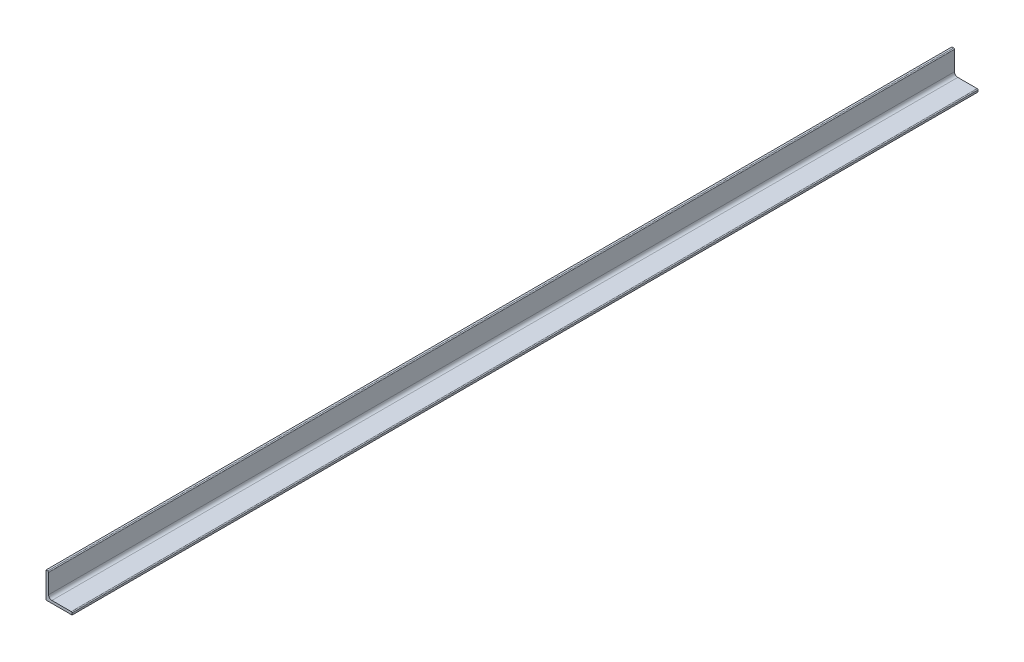
from build123d import *

# Parameters (mm, degrees)
BOSS_EXTRUDE1_DEPTH = 1389


with BuildPart() as part:
    # Sketch1 → Boss-Extrude1 (new body)
    with BuildSketch(Plane.XY):
        with BuildLine():
            Line((0, 0), (0, 40))
            Line((0, 40), (2.666666667, 40))
            ThreePointArc((2.666666667, 40), (3.609475708, 39.609475708), (4, 38.666666667))
            Line((4, 38.666666667), (4, 9))
            ThreePointArc((4, 9), (5.464466094, 5.464466094), (9, 4))
            Line((9, 4), (38.666666667, 4))
            ThreePointArc((38.666666667, 4), (39.609475708, 3.609475708), (40, 2.666666667))
            Line((40, 2.666666667), (40, 0))
            Line((40, 0), (0, 0))
        make_face()
    extrude(amount=BOSS_EXTRUDE1_DEPTH)


solid = part.part
